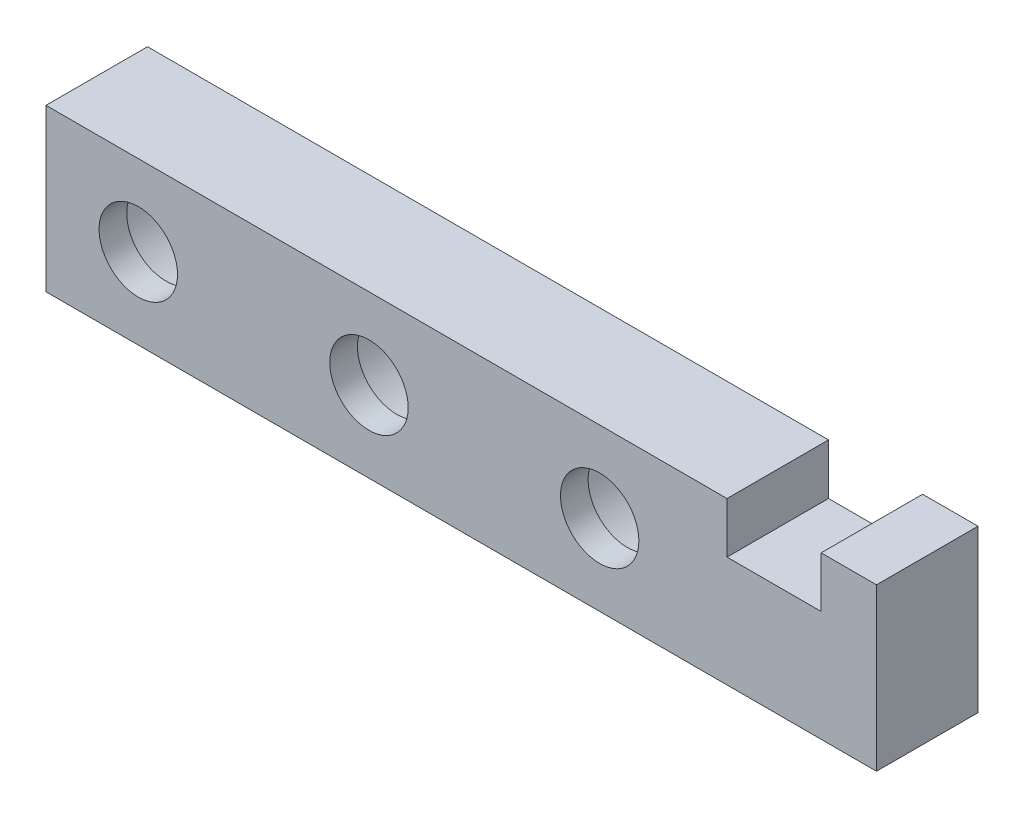
from build123d import *

# Parameters (mm, degrees)
SKETCH1_R           = 4.25
BOSS_EXTRUDE1_DEPTH = 11
CUT_EXTRUDE1_START  = -3
SKETCH2_R           = 7.5
CUT_EXTRUDE1_DEPTH  = 8


with BuildPart() as part:
    # Sketch1 → Boss-Extrude1 (new body)
    with BuildSketch(Plane.XY):
        Polygon((-45, 8.75), (28.8, 8.75), (28.8, 3.25), (39, 3.25), (39, 8.75), (45, 8.75), (45, -8.75), (-45, -8.75), align=None)
        with Locations((-35, 0)):
            Circle(SKETCH1_R, mode=Mode.SUBTRACT)
        with Locations((-10, 0)):
            Circle(SKETCH1_R, mode=Mode.SUBTRACT)
        with Locations((15, 0)):
            Circle(SKETCH1_R, mode=Mode.SUBTRACT)
    extrude(amount=BOSS_EXTRUDE1_DEPTH)

    # Sketch2 → Cut-Extrude1 (cut)
    with BuildSketch(Plane.XY.offset(11).offset(CUT_EXTRUDE1_START)):
        with Locations((-35, 0)):
            Circle(SKETCH2_R)
        with Locations((-10, 0)):
            Circle(SKETCH2_R)
        with Locations((15, 0)):
            Circle(SKETCH2_R)
    extrude(amount=-CUT_EXTRUDE1_DEPTH, mode=Mode.SUBTRACT)


solid = part.part
